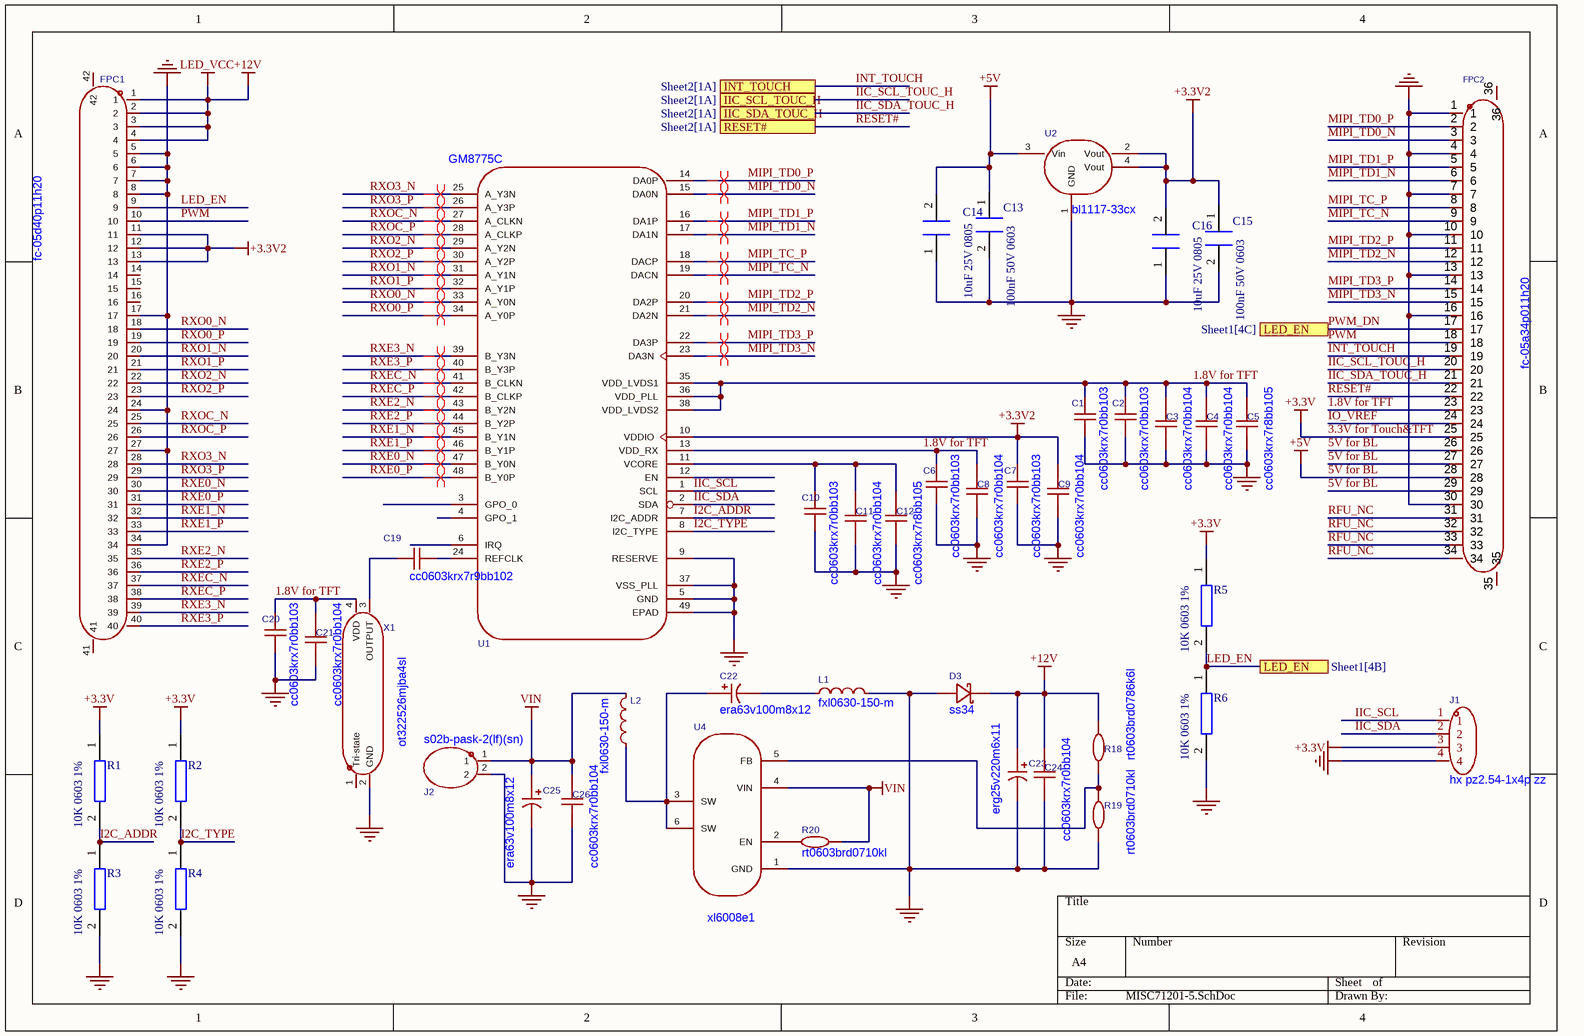
[diagram p0: MISC71201-5.SchDoc]
# Altium project MISC71201-2.PrjPcb
2 sheets, 69 parts. Net scope: flat (ports and power ports of the same name join across sheets).
Board file: MISC71201-3.PcbDoc
Sheets:
  MISC71201-5.SchDoc
  MISC71201-6.SchDoc

## Sheet MISC71201-5.SchDoc
size A4; SheetNumber: 1; SheetTotal: 2

### Parts
C1  cc0603krx7r0bb103  [C0603]
C2  cc0603krx7r0bb103  [C0603]
C3  cc0603krx7r0bb104  [C0603]
C4  cc0603krx7r0bb104  [C0603]
C5  cc0603krx7r8bb105  [C0603]
C6  cc0603krx7r0bb103  [C0603]
C7  cc0603krx7r0bb103  [C0603]
C8  cc0603krx7r0bb104  [C0603]
C9  cc0603krx7r0bb104  [C0603]
C10  cc0603krx7r0bb103  [C0603]
C11  cc0603krx7r0bb104  [C0603]
C12  cc0603krx7r8bb105  [C0603]
C13  100nF 50V 0603  [CAP C0603]
C14  10uF 25V 0805  [CAP C0805]
C15  100nF 50V 0603  [CAP C0603]
C16  10uF 25V 0805  [CAP C0805]
C19  cc0603krx7r9bb102  [C0603]
C20  cc0603krx7r0bb103  [C0603]
C21  cc0603krx7r0bb104  [C0603]
C22  era63v100m8x12  [CAP-TH_BD8.0-P3.50-D0.8-FD]
C23  erg25v220m6x11  [CAP-TH_BD6.3-P2.50-D0.5-FD]
C24  cc0603krx7r0bb104  [C0603]
C25  era63v100m8x12  [CAP-TH_BD8.0-P3.50-D0.8-FD]
C26  cc0603krx7r0bb104  [C0603]
D3  ss34  [SMA_L4.3-W2.6-LS5.0-RD]
FPC1  fc-05d40p11h20  [FPC-SMD_40P-P0.50_FC-05D40P11H20]
FPC2  fc-05a34p011h20  [FPC-SMD_FC-05A34P011H20]
J1  hx pz2.54-1x4p zz  [HDR-TH_4P-P2.54-V-M]
J2  s02b-pask-2(lf)(sn)  [CONN-TH_S02B-PASK-2-LF-SN]
L1  fxl0630-150-m  [IND-SMD_L7.0-W6.6_FXL0630]
L2  fxl0630-150-m  [IND-SMD_L7.0-W6.6_FXL0630]
R1  10K 0603 1%  [RES R0603]
R2  10K 0603 1%  [RES R0603]
R3  10K 0603 1%  [RES R0603]
R4  10K 0603 1%  [RES R0603]
R5  10K 0603 1%  [RES R0603]
R6  10K 0603 1%  [RES R0603]
R18  rt0603brd0786k6l  [R0603]
R19  rt0603brd0710kl  [R0603]
R20  rt0603brd0710kl  [R0603]
U1  GM8775C  [UFQFPN-48_L7.0-W7.0-P0.50-BL-EP]
U2  bl1117-33cx  [SOT-223_L6.5-W3.5-P2.30-LS7.0-BR]
U4  xl6008e1  [TO-252-5_L6.6-W5.8-P1.27-TL]
X1  ot322526mjba4sl  [OSC-SMD_4P-L3.2-W2.5-BL]

### Ports
IIC_SCL_TOUC_H (see Sheet2[1A]), IIC_SDA_TOUC_H (see Sheet2[1A]), INT_TOUCH (see Sheet2[1A]), LED_EN (see Sheet1[4B]), LED_EN (see Sheet1[4C]), RESET# (see Sheet2[1A])

### Nets
3.3V for Touch&TFT: FPC2.25 J1.3 R1.1 R2.1 R5.1  [also labelled +3.3V]
5V for BL: C13.1 C14.2 FPC2.26 FPC2.27 FPC2.28 FPC2.29 U2.3(Vin)  [also labelled +5V]
+3.3V2: C7.2 C9.2 C15.1 C16.2 FPC1.11 FPC1.12 FPC1.13 U1.10(VDDIO) U2.2(Vout) U2.4(Vout)
+12V: C23.1 C24.2 D3.1(A) FPC1.1 FPC1.2 FPC1.3 FPC1.4 R18.2  [also labelled LED_VCC]
GND: C1.1 C2.1 C3.1 C4.1 C5.2 C6.1 C7.1 C8.1 C9.1 C10.1 C11.1 C12.2 C13.2 C14.1 C15.2 C16.1 C20.1 C21.1 C23.2 C24.1 C25.2 C26.1 D3.2(K) FPC1.5 FPC1.6 FPC1.7 FPC1.8 FPC1.17 FPC1.24 FPC1.27 FPC1.34 FPC2.1 FPC2.4 FPC2.7 FPC2.10 FPC2.13 FPC2.16 FPC2.30 J1.4 J2.2 L1.2 R3.2 R4.2 R6.2 R19.2 U1.5(GND) U1.9(RESERVE) U1.37(VSS_PLL) U1.49(EPAD) U2.1(GND) U4.1(GND) X1.2(GND)
VIN: C25.1 C26.2 J2.1 L2.2 R20.2 U4.4(VIN)
1.8V for TFT: C1.2 C2.2 C3.2 C4.2 C5.1 C6.2 C8.2 C20.2 C21.2 FPC2.23 U1.13(VDD_RX) U1.35(VDD_LVDS1) U1.36(VDD_PLL) U1.38(VDD_LVDS2) X1.4(VDD)
I2C_ADDR: R1.2 R3.1 U1.7(I2C_ADDR)
I2C_TYPE: R2.2 R4.1 U1.8(I2C_TYPE)
IIC_SCL: J1.1 U1.1(SCL)
IIC_SCL_TOUC_H: FPC2.20 ; port IIC_SCL_TOUC_H
IIC_SDA: J1.2 U1.2(SDA)
IIC_SDA_TOUC_H: FPC2.21 ; port IIC_SDA_TOUC_H
INT_TOUCH: FPC2.19 ; port INT_TOUCH
IO_VREF: FPC2.24
LED_EN: FPC1.9 FPC2.17 R5.2 R6.1 ; port LED_EN  [also labelled PWM_DN]
MIPI_TC_N: FPC2.9 U1.19(DACN)
MIPI_TC_P: FPC2.8 U1.18(DACP)
MIPI_TD0_N: FPC2.3 U1.15(DA0N)
MIPI_TD0_P: FPC2.2 U1.14(DA0P)
MIPI_TD1_N: FPC2.6 U1.17(DA1N)
MIPI_TD1_P: FPC2.5 U1.16(DA1P)
MIPI_TD2_N: FPC2.12 U1.21(DA2N)
MIPI_TD2_P: FPC2.11 U1.20(DA2P)
MIPI_TD3_N: FPC2.15 U1.23(DA3N)
MIPI_TD3_P: FPC2.14 U1.22(DA3P)
PWM: FPC1.10 FPC2.18
RESET#: FPC2.22 ; port RESET#
RFU_NC: FPC2.31 FPC2.32 FPC2.33 FPC2.34
RXE0_N: FPC1.30 U1.47(B_Y0N)
RXE0_P: FPC1.31 U1.48(B_Y0P)
RXE1_N: FPC1.32 U1.45(B_Y1N)
RXE1_P: FPC1.33 U1.46(B_Y1P)
RXE2_N: FPC1.35 U1.43(B_Y2N)
RXE2_P: FPC1.36 U1.44(B_Y2P)
RXE3_N: FPC1.39 U1.39(B_Y3N)
RXE3_P: FPC1.40 U1.40(B_Y3P)
RXEC_N: FPC1.37 U1.41(B_CLKN)
RXEC_P: FPC1.38 U1.42(B_CLKP)
RXO0_N: FPC1.18 U1.33(A_Y0N)
RXO0_P: FPC1.19 U1.34(A_Y0P)
RXO1_N: FPC1.20 U1.31(A_Y1N)
RXO1_P: FPC1.21 U1.32(A_Y1P)
RXO2_N: FPC1.22 U1.29(A_Y2N)
RXO2_P: FPC1.23 U1.30(A_Y2P)
RXO3_N: FPC1.28 U1.25(A_Y3N)
RXO3_P: FPC1.29 U1.26(A_Y3P)
RXOC_N: FPC1.25 U1.27(A_CLKN)
RXOC_P: FPC1.26 U1.28(A_CLKP)
NetC10_2: C10.2 C11.2 C12.1 U1.11(VCORE)
NetC19_1: C19.1 U1.24(REFCLK)
NetC19_2: C19.2 X1.3(OUTPUT)
NetC22_1: C22.1 L2.1 U4.3(SW) U4.6(SW)
NetC22_2: C22.2 L1.1
NetR18_1: R18.1 R19.1 U4.5(FB)
NetR20_1: R20.1 U4.2(EN)

Not connected (* = marked no-connect by the designer): FPC1 14 15 16 41 42; FPC2 35 36; U1 3(GPO_0) 4(GPO_1) 6(IRQ) 12(EN); X1 1(Tri-state)

### Layout directives
differential pair: MIPI_TC_N, MIPI_TC_P, MIPI_TD0_N, MIPI_TD0_P, MIPI_TD1_N, MIPI_TD1_P, MIPI_TD2_N, MIPI_TD2_P, MIPI_TD3_N, MIPI_TD3_P, RXE0_N, RXE0_P, RXE1_N, RXE1_P, RXE2_N, RXE2_P, RXE3_N, RXE3_P, RXEC_N, RXEC_P, RXO0_N, RXO0_P, RXO1_N, RXO1_P, RXO2_N, RXO2_P, RXO3_N, RXO3_P, RXOC_N, RXOC_P

### Library data of the parts
C1 C2 C6 C7 C10 C20 = cc0603krx7r0bb103: Capacitance:10nF;Tolerance:±10%;Rated voltage:100V;Temp. coefficient:X7R;; Manufacturer: YAGEO(国巨); AddInBom: yes; ModelId: ac125912035d415993ca9572d50418b1; ModelName: C0603_L1.6-W0.8-H0.8; ModelTransform: 62.992,31.496,0,0,0,0,0,0,0; Value: 10nF; Tolerance: ±10%; Voltage Rating: 100V; Temperature Coefficient: X7R; Symbol: CC0603KRX7R0BB103; LCSC Part Name: 10nF ±10% 100V; SupplierPart: C107059; ManufacturerPart: CC0603KRX7R0BB103; Supplier Footprint: 0603; JLCPCB Part Class: Extended Part; Datasheet: https://item.szlcsc.com/datasheet/CC0603KRX7R0BB103/108275.html; Supplier: LCSC; ConvertToPcb: yes; FootprintName: C0603
C3 C4 C8 C9 C11 C21 C24 C26 = cc0603krx7r0bb104: Capacitance:100nF;Tolerance:±10%;Rated voltage:100V;Temp. coefficient:X7R;; Manufacturer: YAGEO(国巨); AddInBom: yes; ModelId: ac125912035d415993ca9572d50418b1; ModelName: C0603_L1.6-W0.8-H0.8; ModelTransform: 62.992,31.496,0,0,0,0,0,0,0; Value: 100nF; Tolerance: ±10%; Voltage Rating: 100V; Temperature Coefficient: X7R; Symbol: CC0603KRX7R0BB104; LCSC Part Name: 100nF ±10% 100V; SupplierPart: C113803; ManufacturerPart: CC0603KRX7R0BB104; Supplier Footprint: 0603; JLCPCB Part Class: Extended Part; Datasheet: https://item.szlcsc.com/datasheet/CC0603KRX7R0BB104/115039.html; Supplier: LCSC; ConvertToPcb: yes; FootprintName: C0603
C5 C12 = cc0603krx7r8bb105: Capacitance:1uF;Tolerance:±10%;Rated voltage:25V;Temp. coefficient:X7R;; Manufacturer: YAGEO(国巨); AddInBom: yes; ModelId: ac125912035d415993ca9572d50418b1; ModelName: C0603_L1.6-W0.8-H0.8; ModelTransform: 62.992,31.496,0,0,0,0,0,0,0; Value: 1uF; Tolerance: ±10%; Voltage Rating: 25V; Temperature Coefficient: X7R; Symbol: CC0603KRX7R8BB105; LCSC Part Name: 1uF ±10% 25V; SupplierPart: C106858; ManufacturerPart: CC0603KRX7R8BB105; Supplier Footprint: 0603; JLCPCB Part Class: Extended Part; Datasheet: https://item.szlcsc.com/datasheet/CC0603KRX7R8BB105/108074.html; Supplier: LCSC; ConvertToPcb: yes; FootprintName: C0603
C13-C16 = CAPACITOR CER
C19 = cc0603krx7r9bb102: Capacitance:1nF;Tolerance:±10%;Rated voltage:50V;Material (temp. coefficient):X7R;; Manufacturer: YAGEO(国巨); AddInBom: yes; ModelId: ac125912035d415993ca9572d50418b1; ModelName: C0603_L1.6-W0.8-H0.8; ModelTransform: 62.992,31.496,0,0,0,0,0,0,0; Value: 1nF; Tolerance: ±10%; Voltage Rated: 50V; Temperature Coefficient: X7R; Symbol: CC0603KRX7R9BB102; LCSC Part Name: 1nF ±10% 50V; SupplierPart: C100040; ManufacturerPart: CC0603KRX7R9BB102; Supplier Footprint: 0603; JLCPCB Part Class: Extended Part; Datasheet: https://atta.szlcsc.com/upload/public/pdf/source/20180910/C282072_33301C7F631E79921B82A8DAC6BCC5B3.pdf; Supplier: LCSC; ConvertToPcb: yes; FootprintName: C0603
C22 C25 = era63v100m8x12: Capacitance:100uF;Tolerance:±20%;Rated voltage:63V;Ripple current:215mA@120Hz;Equivalent series resistance (ESR):-;; Manufacturer: JIERR(捷而瑞); AddInBom: yes; ModelId: bbca4ff951b846bd8e724d96ce125d88; ModelTransform: 315.3537,315.30354,0,0,0,0,0,0,-196.85; Value: 100uF; Tolerance: ±20%; Voltage Rating: 63V; Pin Spacing: 3.5mm; Lifetime: 2000hrs@105℃; Symbol: ERA63V100M8X12; LCSC Part Name: 100uF ±20% 63V; SupplierPart: C49256821; ManufacturerPart: ERA63V100M8X12; Supplier Footprint: 插件,D8xL12mm; JLCPCB Part Class: Extended Part; Datasheet: https://item.szlcsc.com/datasheet/ERA63V100M8X12/51692221.html; Supplier: LCSC; ConvertToPcb: yes; FootprintName: CAP-TH_BD8.0-P3.50-D0.8-FD; ModelName: CAP-TH_BD8.0-P3.50-D0.8-FD; Ripple Current: 215mA@120Hz; Equivalent Series Resistance(ESR): -; Diameter: 8mm; Height - Seated (Max): 12mm; Operating Temperature: -40℃~+105℃
C23 = erg25v220m6x11: Capacitance:220uF;Tolerance:±20%;Rated voltage:25V;Ripple current:510mA@100kHz;Equivalent series resistance (ESR):130mΩ@100kHz;; Manufacturer: JIERR(捷而瑞); AddInBom: yes; ModelId: 983aa343eddc42b59ebb10541a88166e; ModelTransform: 247.99486,248.229,0,90,0,0,0,0,-196.85; Value: 220uF; Tolerance: ±20%; Voltage Rating: 25V; Pin Spacing: 2.5mm; Lifetime: 2000hrs@105℃; Symbol: ERG25V220M6X11; LCSC Part Name: 220uF ±20% 25V; SupplierPart: C47344177; ManufacturerPart: ERG25V220M6X11; Supplier Footprint: 插件,D6.3xL11mm; JLCPCB Part Class: Extended Part; Datasheet: https://item.szlcsc.com/datasheet/ERG25V220M6X11/49556618.html; Supplier: LCSC; ConvertToPcb: yes; FootprintName: CAP-TH_BD6.3-P2.50-D0.5-FD; ModelName: CAP-TH_BD6.3-P2.50-D0.5-FD; Ripple Current: 510mA@100kHz; Equivalent Series Resistance(ESR): 130mΩ@100kHz; Diameter: 6mm; Height - Seated (Max): 11mm; Operating Temperature: -40℃~+105℃
D3 = ss34_c7420365: Diode configuration:Single;Forward voltage (Vf):550mV@3A;DC reverse voltage (Vr):40V;Rectified current:3A;; Manufacturer: R+O(宏嘉诚); AddInBom: yes; ModelId: 7e24bebe6cd74171ae8c9de6fc5b78aa; ModelName: SMA_L4.3-W2.6-LS5.0-FD; ModelTransform: 198.4248,103.5431,0,180,0,0,-0.001,0,0; Diode Configuration: Single; Voltage - DC Reverse(Vr): 40V; Current - Rectified: 3A; Reverse Leakage Current (Ir): 200uA@40V; Symbol: SS34_C7420365; LCSC Part Name: 电压:40V 电流:3A; SupplierPart: C7420365; ManufacturerPart: SS34; Supplier Footprint: SMA(DO-214AC); JLCPCB Part Class: Extended Part; Datasheet: https://item.szlcsc.com/datasheet/SS34/8397187.html; Supplier: LCSC; ConvertToPcb: yes; FootprintName: SMA_L4.3-W2.6-LS5.0-FD; Voltage - Forward(Vf@If): 550mV@3A
FPC1 = fc-05d40p11h20: Locking:Slide;Contact type:Bottom;Contacts:40P;Pitch:0.5mm;Mounting:Horizontal SMT;Operating temperature:-25℃~+85℃;; Manufacturer: BXCONN(宝讯); AddInBom: yes; ModelId: 3b8b2a1f2ab84f5589e4909d5c4b9331; ModelTransform: 1007.872,226.378,0,0,0,0,0,-56.85,0; Locking Feature: Slide; Number of Contacts: 40P; Pitch: 0.5mm; FFC, FCB Thickness: 0.3mm; Rated Voltage (Max): 50V; FPC/FFC Lock: Without latch; Forward Foot / Back Foot: No front/back distinction; Symbol: FC-05D40P11H20; LCSC Part Name: 间距:0.5mm 40P 抽屉式 下接; SupplierPart: C23398806; ManufacturerPart: FC-05D40P11H20; Supplier Footprint: SMD,P=0.5mm,卧贴; JLCPCB Part Class: Extended Part; Datasheet: https://item.szlcsc.com/datasheet/FC-05D40P11H20/25128447.html; Supplier: LCSC; ConvertToPcb: yes; FootprintName: FPC-SMD_40P-P0.50_FC-05D40P11H20; ModelName: FPC-SMD_40P-P0.50_FC-05D40P11H20; Contact Type: Bottom; Mounting Type: Horizontal SMT; Height Above Board: 2mm; Contact Material: Copper alloy; Contact Plating: Tin; Operating Temperature: -25℃~+85℃
FPC2 = fc-05a34p011h20: Locking:Flip;Contact type:Bottom;Contacts:34P;Pitch:0.5mm;Mounting:Horizontal SMT;Operating temperature:-40℃~+85℃;; Manufacturer: BXCONN(宝讯); AddInBom: yes; Locking Feature: Flip; Number of Contacts: 34P; Pitch: 0.5mm; FFC, FCB Thickness: 0.3mm; Rated Voltage (Max): 50V; Current Rating (Max): 500mA; FPC/FFC Lock: Without latch; Forward Foot / Back Foot: No front/back distinction; LCSC Part Name: FPC 翻盖式 下接 P数:34P 间距:0.5mm; SupplierPart: C55079459; ManufacturerPart: FC-05A34P011H20; Supplier Footprint: SMD,P=0.5mm,卧贴; JLCPCB Part Class: Extended Part; Datasheet: https://item.szlcsc.com/datasheet/FC-05A34P011H20/58723328.html; Supplier: LCSC; ConvertToPcb: yes; SymbolName: FC-05A34P011H20; FootprintName: FPC-SMD_FC-05A34P011H20; Contact Type: Bottom; Mounting Type: Horizontal SMT; Height Above Board: 2mm; Contact Material: Phosphor bronze; Contact Plating: Tin; Operating Temperature: -40℃~+85℃
J1 = hx pz2.54-1x4p zz: Pin structure:1x4P;Pitch:2.54mm;Row pitch:-;Round/square pin:Square;Mounting:THT;Rows:Single;Total pins:4P;Rated current:3A;Rated voltage:1kV;Mating pin length:6mm;Insulator height:2.5mm;Tail length:3mm;Contact material:Brass;Contact plating:Gold;Operating temperature:-40℃~+105℃;Color:Black;; Manufacturer: hanxia(韩下); AddInBom: yes; ModelId: 112f4d05e8d64e99ab9a333894bea4f9; ModelName: HDR-TH_4P-P2.54-M-LI-1X4P; ModelTransform: 399.999,104.7242,0,0,0,0,0,0,-118.11; Pin Structure: 1x4P; Pitch: 2.54mm; Current Rating: 3A; Voltage Rating (Max): 1kV; Symbol: HX PZ2.54-1X4P ZZ; LCSC Part Name: 1x4P 间距:2.54mm 方针 直插; SupplierPart: C32713270; ManufacturerPart: HX PZ2.54-1x4P ZZ; Supplier Footprint: 插件,P=2.54mm; JLCPCB Part Class: Extended Part; Datasheet: https://item.szlcsc.com/datasheet/HX%2520PZ2.54-1x4P%2520ZZ/34444550.html; Supplier: LCSC; ConvertToPcb: yes; FootprintName: HDR-TH_4P-P2.54-V-M; Row Spacing: -; Circluar Pins/Square Pins: Square pin; Mounting Type: THT; Number of Rows: Single row; Number of Pins: 4P; Length of Mating Pin: 6mm; Insulation Height: 2.5mm; Length of End Connection Pin: 3mm; Contact Material: Brass; Contact Plating: Gold; Operating Temperature: -40℃~+105℃; Color: Black; Supplementary Features: -
J2 = s02b-pask-2(lf)(sn): Pin structure:1x2P;Pitch:2mm;Mounting:Right-angle THT;Series:PA;Total pins:2P;Rows:1;Pins per row:2;Row pitch:-;Rated current:3A;Contact material:Copper alloy;Contact plating:Tin;Operating temperature:-25℃~+85℃;; Manufacturer: JST; AddInBom: yes; ModelId: 2337b366cde64323a694946c54673667; ModelTransform: 236.22,460.629,0,0,0,0,0,93.11,-137.795; Pins Structure: 1x2P; Pitch: 2mm; Reference Series: PA; Number of PINs Per Row: 2; Current Rating: 3A; Voltage Rating: 250V; Plastic Material: Glass-fibre reinforced PBT; Flame Retardant Rating: UL94V-0; Supplementary Features: With post; K-type pins; Z-Height of the Board: 6.5mm; X-Length of Bottom Edge on Board (Spacing Line): 6mm; Y-Width of Bottom Edge on Board: 11.7mm; Symbol: S02B-PASK-2(LF)(SN); LCSC Part Name: 1x2P 间距:2mm 弯插 系列:PA; SupplierPart: C265094; ManufacturerPart: S02B-PASK-2(LF)(SN); Supplier Footprint: 弯插,P=2mm; JLCPCB Part Class: Extended Part; Datasheet: https://item.szlcsc.com/datasheet/S02B-PASK-2(LF)(SN)/255465.html; Supplier: LCSC; ConvertToPcb: yes; FootprintName: CONN-TH_S02B-PASK-2-LF-SN; ModelName: CONN-TH_S02B-PASK-2-LF-SN; Mounting Type: Right-angle THT; Number of Pins: 2P; Number of Rows: 1; Row Spacing: -; Contact Material: Copper alloy; Contact Plating: Tin; Operating Temperature: -25℃~+85℃; Color: White
L1 L2 = fxl0630-150-m: SMD, 7x6.6x2.8mm   alloy inductor, molded inductor, high current; Manufacturer: cjiang(长江微电); AddInBom: yes; ModelId: 6712504104d74f0ca01cd7d0df9965b7; ModelName: IND-SMD_L7.0-W6.6-H2.8_FXL0630; ModelTransform: 275.59,259.842,0,0,0,0,0,0,0; Symbol: FXL0630-150-M; LCSC Part Name: 15uH ±20%; SupplierPart: C177243; ManufacturerPart: FXL0630-150-M; Supplier Footprint: SMD,7x6.6mm; JLCPCB Part Class: Extended Part; Datasheet: https://item.szlcsc.com/datasheet/FXL0630-150-M/188635.html; Supplier: LCSC; ConvertToPcb: yes; FootprintName: IND-SMD_L7.0-W6.6_FXL0630
R1-R6 = Resistor
R18 = rt0603brd0786k6l: Resistor type:Thin film;Resistance:86.6kΩ;Tolerance:±0.1%;Power:100mW;Temp. coefficient:±25ppm/℃;; Manufacturer: YAGEO(国巨); AddInBom: yes; ModelId: fc143cca1e79419f9cd78b61e9279f08; ModelTransform: 31.8897,63.7794,0,90,0,0,0,0,0; Value: 86.6kΩ; Tolerance: ±0.1%; Power(Watts): 100mW; Symbol: RT0603BRD0786K6L; LCSC Part Name: 薄膜电阻 86.6kΩ ±0.1% 100mW; SupplierPart: C861580; ManufacturerPart: RT0603BRD0786K6L; Supplier Footprint: 0603; JLCPCB Part Class: Extended Part; Datasheet: https://atta.szlcsc.com/upload/public/pdf/source/20200610/C326738_5639A9F1B6EB6E4AE2197577D3456E7F.pdf; Supplier: LCSC; ConvertToPcb: yes; FootprintName: R0603; ModelName: R0603; Type: Thin film resistor; Temperature Coefficient: ±25ppm/℃; Operating Temperature Range: -55℃~+155℃
R19 R20 = rt0603brd0710kl: Resistor type:Thin film;Resistance:10kΩ;Tolerance:±0.1%;Power:100mW;Operating voltage:75V;Temp. coefficient:±25ppm/℃;; Manufacturer: YAGEO(国巨); AddInBom: yes; ModelId: fc143cca1e79419f9cd78b61e9279f08; ModelTransform: 31.8897,63.7794,0,90,0,0,0,0,0; Value: 10kΩ; Tolerance: ±0.1%; Power(Watts): 100mW; Voltage-Supply(Max): 75V; Symbol: RT0603BRD0710KL; LCSC Part Name: 薄膜电阻 10kΩ ±0.1% 100mW; SupplierPart: C95204; ManufacturerPart: RT0603BRD0710KL; Supplier Footprint: 0603; JLCPCB Part Class: Extended Part; Datasheet: https://item.szlcsc.com/datasheet/RT0603BRD0710KL/96405.html; Supplier: LCSC; ConvertToPcb: yes; FootprintName: R0603; ModelName: R0603; Type: Thin film resistor; Temperature Coefficient: ±25ppm/℃; Operating Temperature: -55℃~+155℃
U1 = stm32f411ceu6: CPU core:ARM Cortex-M4;CPU max frequency:100MHz;CPU bits:32 Bit;; Manufacturer: ST(意法半导体); AddInBom: yes; ModelId: 726e846686ee4a71b91fd16fb4ca286d; ModelName: UFQFPN-48_L7.0-W7.0-H0.6-P0.50; ModelTransform: 275.591,275.59,0,90,0,0,0,0,0; CPU Maximum Speed: 100MHz; Core Size: 32 Bit; Program Storage Size: 512KB; Program Memory Type: FLASH; RAM Size: 128KB; Number of I/O: 36; ADC (Bit): 12bit; Oscillator Type: Built-in; Voltage - Supply: 1.7V~3.6V; Symbol: STM32F411CEU6; LCSC Part Name: 带DSP和FPU的高性能基本型系列ARM Cortex-M4 MCU，具有512 KB Flash、100 MHz CPU和ART加速器; SupplierPart: C60420; ManufacturerPart: STM32F411CEU6; Supplier Footprint: UFQFPN-48(7x7); JLCPCB Part Class: Extended Part; Datasheet: https://item.szlcsc.com/datasheet/STM32F411CEU6/61472.html; Supplier: LCSC; ConvertToPcb: yes; FootprintName: UFQFPN-48_L7.0-W7.0-P0.50-BL-EP; CPU Core: ARM Cortex-M4; EEPROM: -; Operating Temperature: -40℃~+85℃
U2 = bl1117-33cx: Output polarity:Positive;Operating voltage:12V;Output voltage:3.3V;Output current:1A;PSRR:60dB@(120Hz);Output type:Fixed;; Manufacturer: BL(上海贝岭); AddInBom: yes; ModelId: 925194bf9823436183a3e0b978a8d076; ModelName: SOT-223-4P_L6.5-W3.5-H1.6-LS7.0-P2.30; ModelTransform: 279.89794,255.905,0,180,0,0,-0.0005,-0.0005,0; Voltage - Supply: 12V; Output Voltage: 3.3V; Output Current: 1A; Voltage Dropout: 1.5V@(1A); standby current: 2mA; Output Type: Fixed; Number of Outputs: 1; Symbol: BL1117-33CX; LCSC Part Name: 3.3V 1A 12V; SupplierPart: C5400; ManufacturerPart: BL1117-33CX; Supplier Footprint: SOT-223; JLCPCB Part Class: Extended Part; Datasheet: https://item.szlcsc.com/datasheet/BL1117-33CX/5838.html; Supplier: LCSC; ConvertToPcb: yes; FootprintName: SOT-223-4_L6.5-W3.5-P2.30-LS7.0-BR; Output Configuration: Positive; Power Supply Rejection Ratio (PSRR): 60dB@(120Hz); Noise: -; Features: Thermal shutdown; Overcurrent protection; Operating Temperature: -20℃~+125℃@(Tj)
U4 = xl6008e1: Function:Buck-boost;Operating voltage:3.6V~32V;Output voltage:-;Output current:3A;Output type:Adjustable;; Manufacturer: XLSEMI(芯龙); Symbol: XL6008E1_C73012; AddInBom: yes; ModelId: 93fed583f6f249ed8c4cbd02c90976fc; ModelName: TO-252-5_L6.5-W5.6-H2.3-LS9.8-P1.27; ModelTransform: 255.905,386.34112,0,270,0,0,39.37,0,0; Output Current: 3A; Frequency - Switching: 320kHz~480kHz; Synchronous Rectifier: No; Number of Outputs: 1; Topology: Inverting; Boost; SEPIC; Flyback; Quiescent Current: 2.5mA; Switch tube (built-in/external): Built-in; LCSC Part Name: 升降压型 3A 3.6V~32V; SupplierPart: C73012; ManufacturerPart: XL6008E1; Supplier Footprint: TO-252-5; JLCPCB Part Class: Extended Part; Datasheet: https://item.szlcsc.com/datasheet/XL6008E1/74125.html; Supplier: LCSC; ConvertToPcb: yes; FootprintName: TO-252-5_L6.6-W5.8-P1.27-TL; Function: Buck-boost; Voltage - Supply: 3.6V~32V; Output Voltage: -; Operating Temperature: -40℃~+125℃@(TJ); Output Type: Adjustable; Features: Overcurrent protection
X1 = ot322526mjba4sl: Frequency:26MHz;Frequency tolerance (room temp.):±10ppm;Output:CMOS;Operating voltage:1.8V~3.3V;Frequency stability:±20ppm;; Manufacturer: YXC(扬兴晶振); AddInBom: yes; ModelId: ae22b8d143894765bc8100c37cb6356f; ModelName: OSC-SMD_4P-L3.2-W2.5-H1.0; ModelTransform: 125.984,98.425,0,0,0,0,0,0,0; Value: 26MHz; Normal temperature Frequency Tolerance: ±10ppm; Output Type: CMOS; Frequency Stability: ±20ppm; Symbol: OT322526MJBA4SL; LCSC Part Name: YSO110TR 26MHZ 1.8V-3.3V ±10PPM -40~85℃（±20PPM) CMOS; SupplierPart: C4353708; ManufacturerPart: OT322526MJBA4SL; Supplier Footprint: SMD3225-4P; JLCPCB Part Class: Extended Part; Datasheet: https://item.szlcsc.com/datasheet/OT322526MJBA4SL/4924207.html; Supplier: LCSC; ConvertToPcb: yes; FootprintName: OSC-SMD_4P-L3.2-W2.5-BL; Voltage - Supply: 1.8V~3.3V; Operating Temperature: -40℃~+85℃

## Sheet MISC71201-6.SchDoc
size A4; SheetNumber: 2; SheetTotal: 2
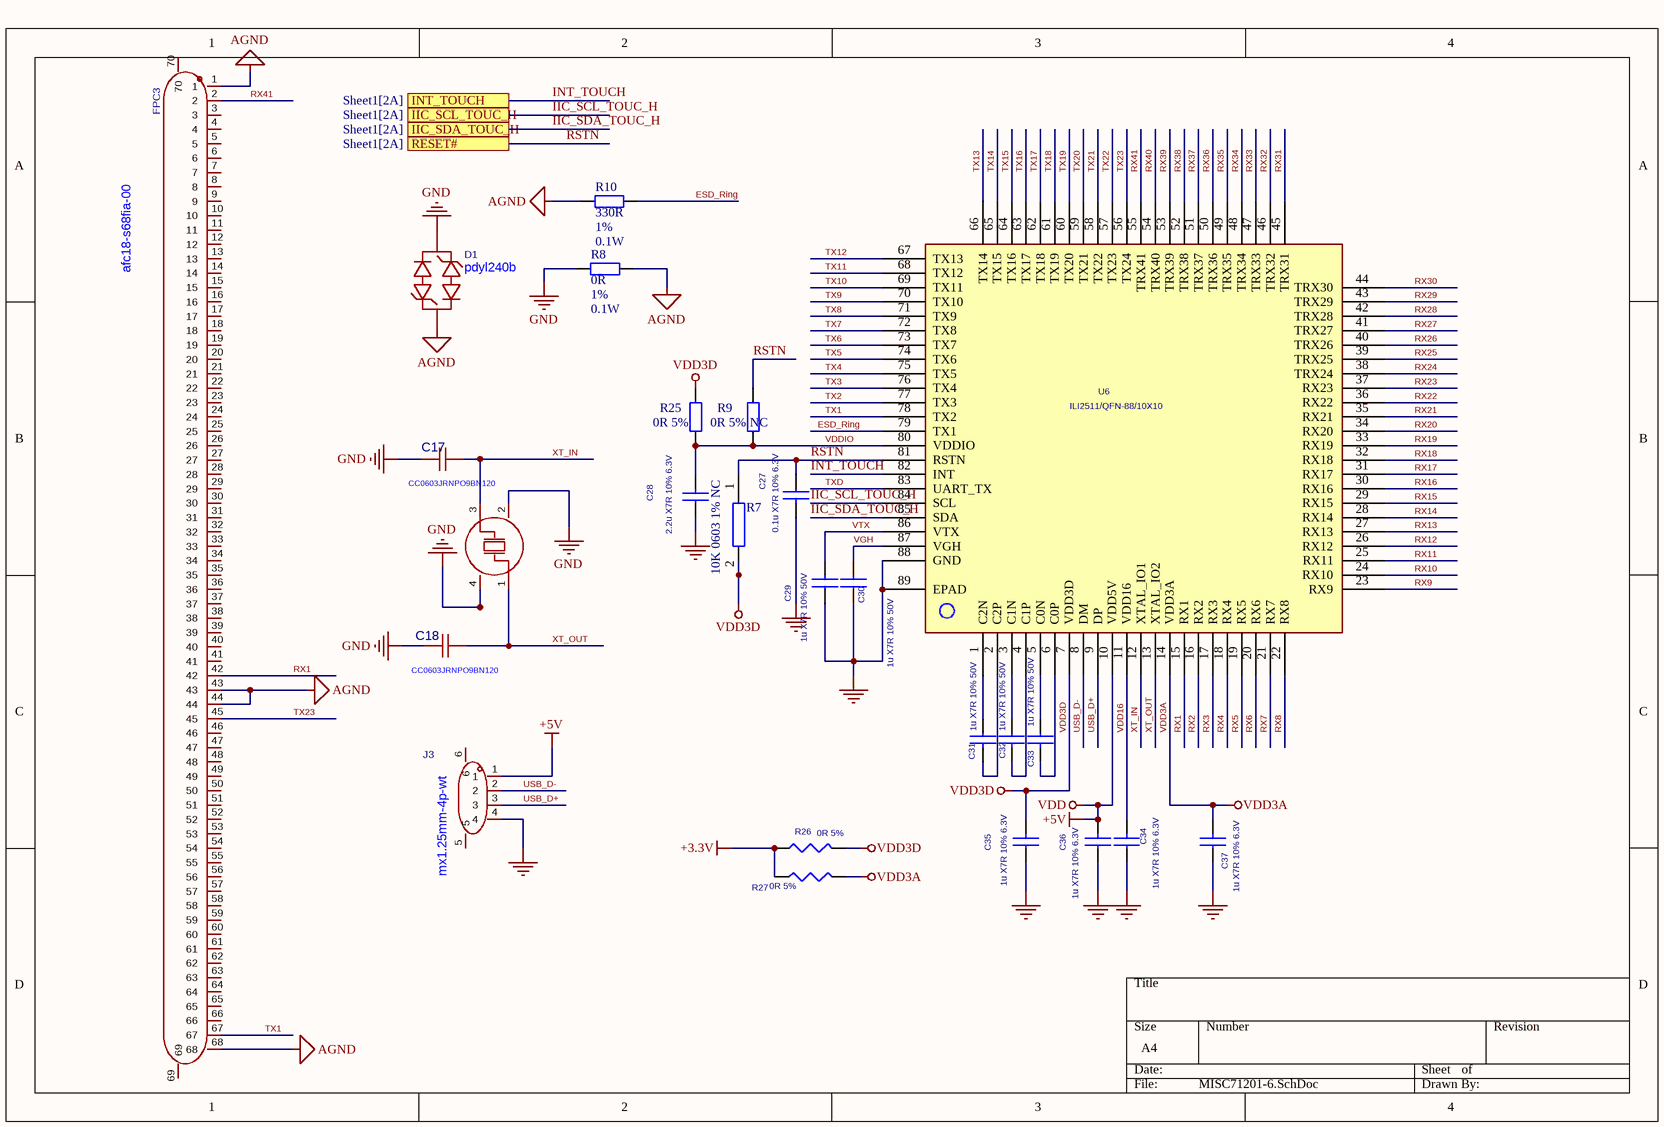
[diagram p1: MISC71201-6.SchDoc]

### Parts
C17  CC0603JRNPO9BN120  [CAP C0603]
C18  CC0603JRNPO9BN120  [CAP C0603]
C27  0.1u X7R 10% 6.3V  [C0603]
C28  2.2u X7R 10% 6.3V  [C0603]
C29  1u X7R 10% 50V  [C0603]
C30  1u X7R 10% 50V  [C0603]
C31  1u X7R 10% 50V  [C0603]
C32  1u X7R 10% 50V  [C0603]
C33  1u X7R 10% 50V  [C0603]
C34  1u X7R 10% 6.3V  [C0603]
C35  1u X7R 10% 6.3V  [C0603]
C36  1u X7R 10% 6.3V  [C0603]
C37  1u X7R 10% 6.3V  [C0603]
D1  pdyl240b  [SOD-323_L1.8-W1.3-LS2.5-RD]
FPC3  afc18-s68fia-00  [CONN-SMD_AFC18-S68FIA-00]
J3  mx1.25mm-4p-wt  [CONN-SMD_MX1.25MM-4P-WT]
R7  10K 0603 1% NC  [RES R0603]
R8  value 0R  TOLERANCE: 1%  POWER: 0.1W  [RES R0603]  (hidden comment: 0R 0603)
R9  0R 5% NC  [R0603]
R10  value 330R  TOLERANCE: 1%  POWER: 0.1W  [RES R0603]  (hidden comment: 0R 0603)
R25  0R 5%  [R0603]
R26  0R 5%  [R0402]
R27  0R 5%  [R0402]
U6  ILI2511/QFN-88/10X10  [ILI2511/QFN-88/10X10]
X2  x322512msb4si  [CRYSTAL-SMD_4P-L3.2-W2.5-BL]  (value not drawn)

### Ports
IIC_SCL_TOUC_H (see Sheet1[2A]), IIC_SDA_TOUC_H (see Sheet1[2A]), INT_TOUCH (see Sheet1[2A]), RESET# (see Sheet1[2A])

### Nets
+3.3V: R26.1 R27.1  [project net 3.3V for Touch&TFT]
+5V: C36.2 J3.1 U6.10(VDD5V)  [also labelled VDD]  [project net 5V for BL]
AGND: D1.2 FPC3.1 FPC3.43 FPC3.44 FPC3.68 R8.2 R10.1
GND: C17.1 C18.1 C27.2 C28.1 C29.1 C30.1 C34.1 C35.1 C36.1 C37.1 D1.1 J3.4 R8.1 U6.88(GND) U6.89(EPAD) X2.2(GND) X2.4(GND)
VDD3A: C37.2 R27.2 U6.14(VDD3A)
VDD3D: C35.2 R7.2 R25.2 R26.2 U6.7(VDD3D)
ESD_Ring: R10.2 U6.79(TX1)
IIC_SCL_TOUC_H: U6.84(SCL) ; port IIC_SCL_TOUC_H
IIC_SDA_TOUC_H: U6.85(SDA) ; port IIC_SDA_TOUC_H
INT_TOUCH: U6.82(INT) ; port INT_TOUCH
RSTN: C27.1 R7.1 R9.2 U6.81(RSTN) ; port RESET#  [project net RESET#]
RX1: FPC3.42 U6.15(RX1)
RX2: U6.16(RX2)
RX3: U6.17(RX3)
RX4: U6.18(RX4)
RX5: U6.19(RX5)
RX6: U6.20(RX6)
RX7: U6.21(RX7)
RX8: U6.22(RX8)
RX9: U6.23(RX9)
RX10: U6.24(RX10)
RX11: U6.25(RX11)
RX12: U6.26(RX12)
RX13: U6.27(RX13)
RX14: U6.28(RX14)
RX15: U6.29(RX15)
RX16: U6.30(RX16)
RX17: U6.31(RX17)
RX18: U6.32(RX18)
RX19: U6.33(RX19)
RX20: U6.34(RX20)
RX21: U6.35(RX21)
RX22: U6.36(RX22)
RX23: U6.37(RX23)
RX24: U6.38(TRX24)
RX25: U6.39(TRX25)
RX26: U6.40(TRX26)
RX27: U6.41(TRX27)
RX28: U6.42(TRX28)
RX29: U6.43(TRX29)
RX30: U6.44(TRX30)
RX31: U6.45(TRX31)
RX32: U6.46(TRX32)
RX33: U6.47(TRX33)
RX34: U6.48(TRX34)
RX35: U6.49(TRX35)
RX36: U6.50(TRX36)
RX37: U6.51(TRX37)
RX38: U6.52(TRX38)
RX39: U6.53(TRX39)
RX40: U6.54(TRX40)
RX41: FPC3.2 U6.55(TRX41)
TX1: FPC3.67 U6.78(TX2)
TX2: U6.77(TX3)
TX3: U6.76(TX4)
TX4: U6.75(TX5)
TX5: U6.74(TX6)
TX6: U6.73(TX7)
TX7: U6.72(TX8)
TX8: U6.71(TX9)
TX9: U6.70(TX10)
TX10: U6.69(TX11)
TX11: U6.68(TX12)
TX12: U6.67(TX13)
TX13: U6.66(TX14)
TX14: U6.65(TX15)
TX15: U6.64(TX16)
TX16: U6.63(TX17)
TX17: U6.62(TX18)
TX18: U6.61(TX19)
TX19: U6.60(TX20)
TX20: U6.59(TX21)
TX21: U6.58(TX22)
TX22: U6.57(TX23)
TX23: FPC3.45 U6.56(TX24)
TXD: U6.83(UART_TX)
USB_D+: J3.3 U6.9(DP)
USB_D-: J3.2 U6.8(DM)
VDD16: C34.2 U6.11(VDD16)
VDDIO: C28.2 R9.1 R25.1 U6.80(VDDIO)
VGH: C30.2 U6.87(VGH)
VTX: C29.2 U6.86(VTX)
XT_IN: C17.2 U6.12(XTAL_IO1) X2.3(OSC2)
XT_OUT: C18.2 U6.13(XTAL_IO2) X2.1(OSC1)
NetC31_1: C31.1 U6.1(C2N)
NetC31_2: C31.2 U6.2(C2P)
NetC32_1: C32.1 U6.3(C1N)
NetC32_2: C32.2 U6.4(C1P)
NetC33_1: C33.1 U6.5(C0N)
NetC33_2: C33.2 U6.6(C0P)

Not connected (* = marked no-connect by the designer): FPC3 3 4 5 6 7 8 9 10 11 12 13 14 15 16 17 18 19 20 21 22 23 24 25 26 27 28 29 30 31 32 33 34 35 36 37 38 39 40 41 46 47 48 49 50 51 52 53 54 55 56 57 58 59 60 61 62 63 64 65 66 69 70; J3 5 6

### Library data of the parts
C17 C18 = CC0603JRNPO9BN120: 12PF; Symbol: CC0603JRNPO9BN120
C27 = C0402_1u_6.3V_X5R: SMD capacitor; PartNumber: 00226021661; Vendor: Faithful LINK; Value2: X5R; Value1: 0.1uF/6.3V
C28 C34-C37 = C0402_2.2u_6.3V_X5R: SMD capacitor; PartNumber: 002260222561; Vendor: Faithful LINK; Value2: X5R; Value1: 1uF/6.3V
C29 C30 = C0603_1u_50V_X7R: SMD capacitor; PartNumber: 002260310544; Value1: 4.7uF/50V; Vendor: Faithful LINK; Value2: X7R
C31-C33 = C0603_1u_50V_X7R: SMD capacitor; PartNumber: 002260310544; Value1: 1uF/50V; Vendor: Faithful LINK; Value2: X7R
D1 = pdyl240b_c5187140: Reverse standoff voltage (Vrwm):24V;Clamping voltage:60V;Peak pulse power (Ppp):350W@8/20us;Breakdown voltage (VBR):26.7V;; Manufacturer: Leiditech(雷卯电子); AddInBom: yes; ModelId: f9eb3c564310447fa7e5a2d35bef3787; ModelName: SOD-323_L1.8-W1.3-LS2.5-BI; ModelTransform: 98.425,51.181,0,0,0,0,0,0,0; Reverse Stand-Off Voltage (Vrwm): 24V; Clamping Voltage: 60V; Voltage - Breakdown: 26.7V; Reverse Leakage Current (Ir): 1uA; level of protection: IEC 61000-4-4；IEC 61000-4-5；IEC 61000-4-2; Type: ESD; Junction Capacitance: 1pF; Symbol: PDYL240B_C5187140; LCSC Part Name: ESD 24V截止; SupplierPart: C5187140; ManufacturerPart: PDYL240B; Supplier Footprint: SOD-323; JLCPCB Part Class: Extended Part; Datasheet: https://item.szlcsc.com/datasheet/PDYL240B/5859019.html; Supplier: LCSC; ConvertToPcb: yes; FootprintName: SOD-323_L1.8-W1.3-LS2.5-BI; Peak Pulse Power Dissipation (Ppp): 350W@8/20us
FPC3 = afc18-s68fia-00: Locking:Flip;Contact type:Bottom;Contacts:68P;Pitch:0.5mm;Mounting:Horizontal SMT;Operating temperature:-25℃~+85℃;; Manufacturer: JS(钜硕电子); AddInBom: yes; ModelId: 3d2b298f609244d39322a05a0bb4d6c8; ModelTransform: 1562.989,195.2752,0,0,0,0,0.001,-38.386,0; Locking Feature: Flip; Number of Contacts: 68P; Pitch: 0.5mm; FFC, FCB Thickness: 0.3mm; Rated Voltage (Max): 50V; Current Rating (Max): 500mA; FPC/FFC Lock: With latch; Forward Foot / Back Foot: No front/back distinction; Symbol: AFC18-S68FIA-00; LCSC Part Name: 翻盖式 下接 P数:68P 间距:0.5mm; SupplierPart: C2842533; ManufacturerPart: AFC18-S68FIA-00; Supplier Footprint: SMD,P=0.5mm,卧贴; JLCPCB Part Class: Extended Part; Datasheet: https://item.szlcsc.com/datasheet/AFC18-S68FIA-00/3027882.html; Supplier: LCSC; ConvertToPcb: yes; FootprintName: CONN-SMD_AFC18-S68FIA-00; ModelName: CONN-SMD_AFC18-S68FIA-00; Contact Type: Bottom; Mounting Type: Horizontal SMT; Height Above Board: 1.78mm; Contact Material: Phosphor bronze; Contact Plating: Gold; Operating Temperature: -25℃~+85℃
J3 = mx1.25mm-4p-wt: Pin structure:1x4P;Pitch:1.25mm;Mounting:Horizontal SMT;Series:PicoBlade(MX 1.25);Total pins:4P;Rows:1;Pins per row:4;Rated current:1A;Contact material:Brass;Contact plating:Tin;Operating temperature:-25℃~+85℃;; Manufacturer: LXWCONN(连兴旺电子); AddInBom: yes; ModelId: a92804599bf0400e8e5e585fff8e0718; ModelTransform: 394.094,206.693,0,0,0,0,-0.005,-28.618,0; Pins Structure: 1x4P; Pitch: 1.25mm; Number of PINs Per Row: 4; Current Rating: 1A; Voltage Rating: 125V; Plastic Material: LCP; Symbol: MX1.25MM-4P-WT; LCSC Part Name: 1x4P 间距:1.25mm 卧贴 系列:PicoBlade(MX 1.25); SupplierPart: C53055350; ManufacturerPart: MX1.25mm-4P-WT; Supplier Footprint: SMD,P=1.25mm,卧贴; JLCPCB Part Class: Extended Part; Datasheet: https://item.szlcsc.com/datasheet/MX1.25mm-4P-WT/55999550.html; Supplier: LCSC; ConvertToPcb: yes; FootprintName: CONN-SMD_MX1.25MM-4P-WT; ModelName: CONN-SMD_MX1.25MM-4P-WT; Mounting Type: Horizontal SMT; Reference Series: PicoBlade(MX 1.25); Number of Pins: 4P; Number of Rows: 1; Contact Material: Brass; Contact Plating: Tin; Operating Temperature: -25℃~+85℃
R7 = Resistor
R8 R10 = Res2: Published: 8-Jun-2000; LatestRevisionDate: 17-Jul-2002; LatestRevisionNote: Re-released for DXP Platform.; PackageReference: AXIAL-0.4; PackageDescription: Axial Device, Thru-Hole; 2 Leads; 0.4 in Pin Spacing; Publisher: Altium Limited
R9 R25 = Res2: SMD resistor; Value: 10K; Published: 8-Jun-2000; LatestRevisionDate: 17-Jul-2002; LatestRevisionNote: Re-released for DXP Platform.; PackageReference: R0603; PackageDescription: Axial Device, Thru-Hole; 2 Leads; 0.4 in Pin Spacing; Publisher: Altium Limited
R26 R27 = R0402_0R_+-5%_Dup2: SMD resistor; PartNumber: 00105020003; Vendor: YAGEO; Value2: ∮5%; Value1: 0R
U6 = ILI2511/QFN-88/10X10_0.4_0.9: ILITEK IC; Part Name: 005122ILI2511; Vendor: ILITEK
X2 = x322512msb4si: Crystal type:SMD crystal;Frequency:12MHz;Frequency tolerance (room temp.):±10ppm;Load capacitance:20pF;Frequency stability:±20ppm;; Manufacturer: YXC(扬兴晶振); AddInBom: yes; ModelId: ff2dfd5650294453a14147960efe1838; ModelTransform: 125.984,98.425,0,0,0,0,0,0,0; Value: 12MHz; Normal temperature Frequency Tolerance: ±10ppm; Load Capacitance: 20pF; Frequency Stability: ±20ppm; Equivalent Series Resistance(ESR): 80Ω; Symbol: X322512MSB4SI; LCSC Part Name: YSX321SL 12MHZ 4P 3225 20PF ±10PPM -40~85℃ (±20PPM); SupplierPart: C9002; ManufacturerPart: X322512MSB4SI; Supplier Footprint: SMD3225-4P; JLCPCB Part Class: Basic Part; Datasheet: https://item.szlcsc.com/datasheet/X322512MSB4SI/9522.html; Supplier: LCSC; ConvertToPcb: yes; FootprintName: CRYSTAL-SMD_4P-L3.2-W2.5-BL; ModelName: CRYSTAL-SMD_4P-L3.2-W2.5-BL; Type: SMD crystal; Operating Temperature: -40℃~+85℃

## Nets that join several sheets
3.3V for Touch&TFT: MISC71201-5 (5 pins), MISC71201-6 (R26.1 R27.1)
5V for BL: MISC71201-5 (7 pins), MISC71201-6 (C36.2 J3.1 U6.10)
GND: MISC71201-5 (52 pins), MISC71201-6 (17 pins)
IIC_SCL_TOUC_H: MISC71201-5 (FPC2.20), MISC71201-6 (U6.84)
IIC_SDA_TOUC_H: MISC71201-5 (FPC2.21), MISC71201-6 (U6.85)
INT_TOUCH: MISC71201-5 (FPC2.19), MISC71201-6 (U6.82)
RESET#: MISC71201-5 (FPC2.22), MISC71201-6 (C27.1 R7.1 R9.2 U6.81)